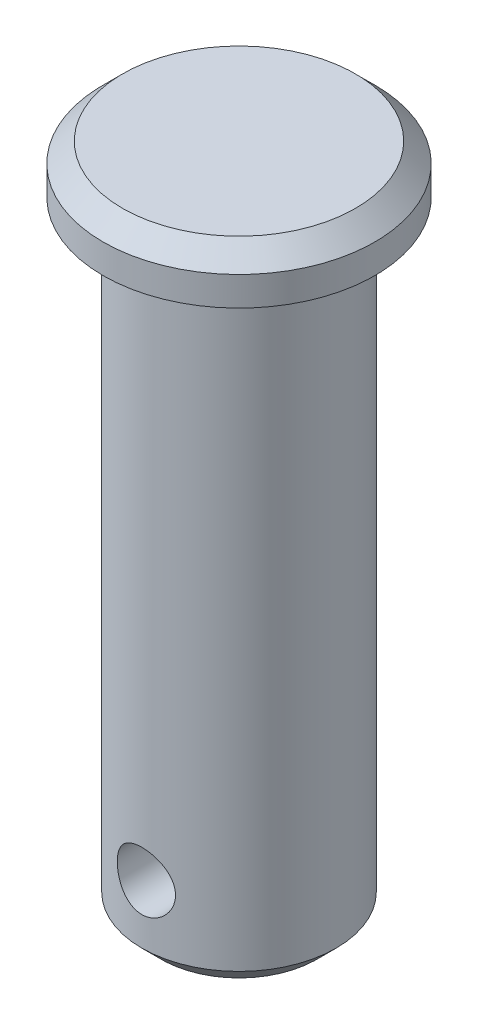
from build123d import *

# Parameters (mm, degrees)
SKETCH_1_R               = 7
EXTRUDE_1_DEPTH          = 2.5
SKETCH_2_R               = 5
EXTRUDE_2_DEPTH          = 32
CHAMFER_1_SIZE           = 1
CUT_EXTRUDE_2_DEPTH      = 34.496268449
CUT_EXTRUDE_2_DEPTH_BACK = 34.496268449
SKETCH_10_R              = 1.5
FILLET_1_R               = 0.5


with BuildPart() as part:
    # 草图1 → 凸台-拉伸1 (new body)
    with BuildSketch(Plane(origin=(0, 0, 0), x_dir=(1, 0, 0), z_dir=(0, 1, 0))):
        with Locations(Location((0, 0, 0), (0, 0, 270))):
            Circle(SKETCH_1_R)
    extrude(amount=EXTRUDE_1_DEPTH)

    # 草图2 → 凸台-拉伸2 (add)
    with BuildSketch(Plane.XZ):
        with Locations(Location((0, 0, 0), (0, 0, 270))):
            Circle(SKETCH_2_R)
    extrude(amount=EXTRUDE_2_DEPTH)

    # 倒角1
    chamfer_1_edges = [part.edges().sort_by_distance(p)[0] for p in [
        (0, 2.5, -7),
        (0, -32, 5),
    ]]
    chamfer(chamfer_1_edges, length=CHAMFER_1_SIZE)

    # 草图10 → 切除-拉伸2 (cut, two sides: drawn at the far end of the back side and taken through both)
    with BuildSketch(Plane.XY.offset(-CUT_EXTRUDE_2_DEPTH_BACK)):
        with Locations(Location((0, -28, 0), (0, 0, 270.000000018))):
            Circle(SKETCH_10_R)
    extrude(amount=CUT_EXTRUDE_2_DEPTH + CUT_EXTRUDE_2_DEPTH_BACK, mode=Mode.SUBTRACT)

    # 圆角1
    fillet_1_edges = [part.edges().sort_by_distance(p)[0] for p in [
        (0, 0, 5),
    ]]
    fillet(fillet_1_edges, radius=FILLET_1_R)


solid = part.part
